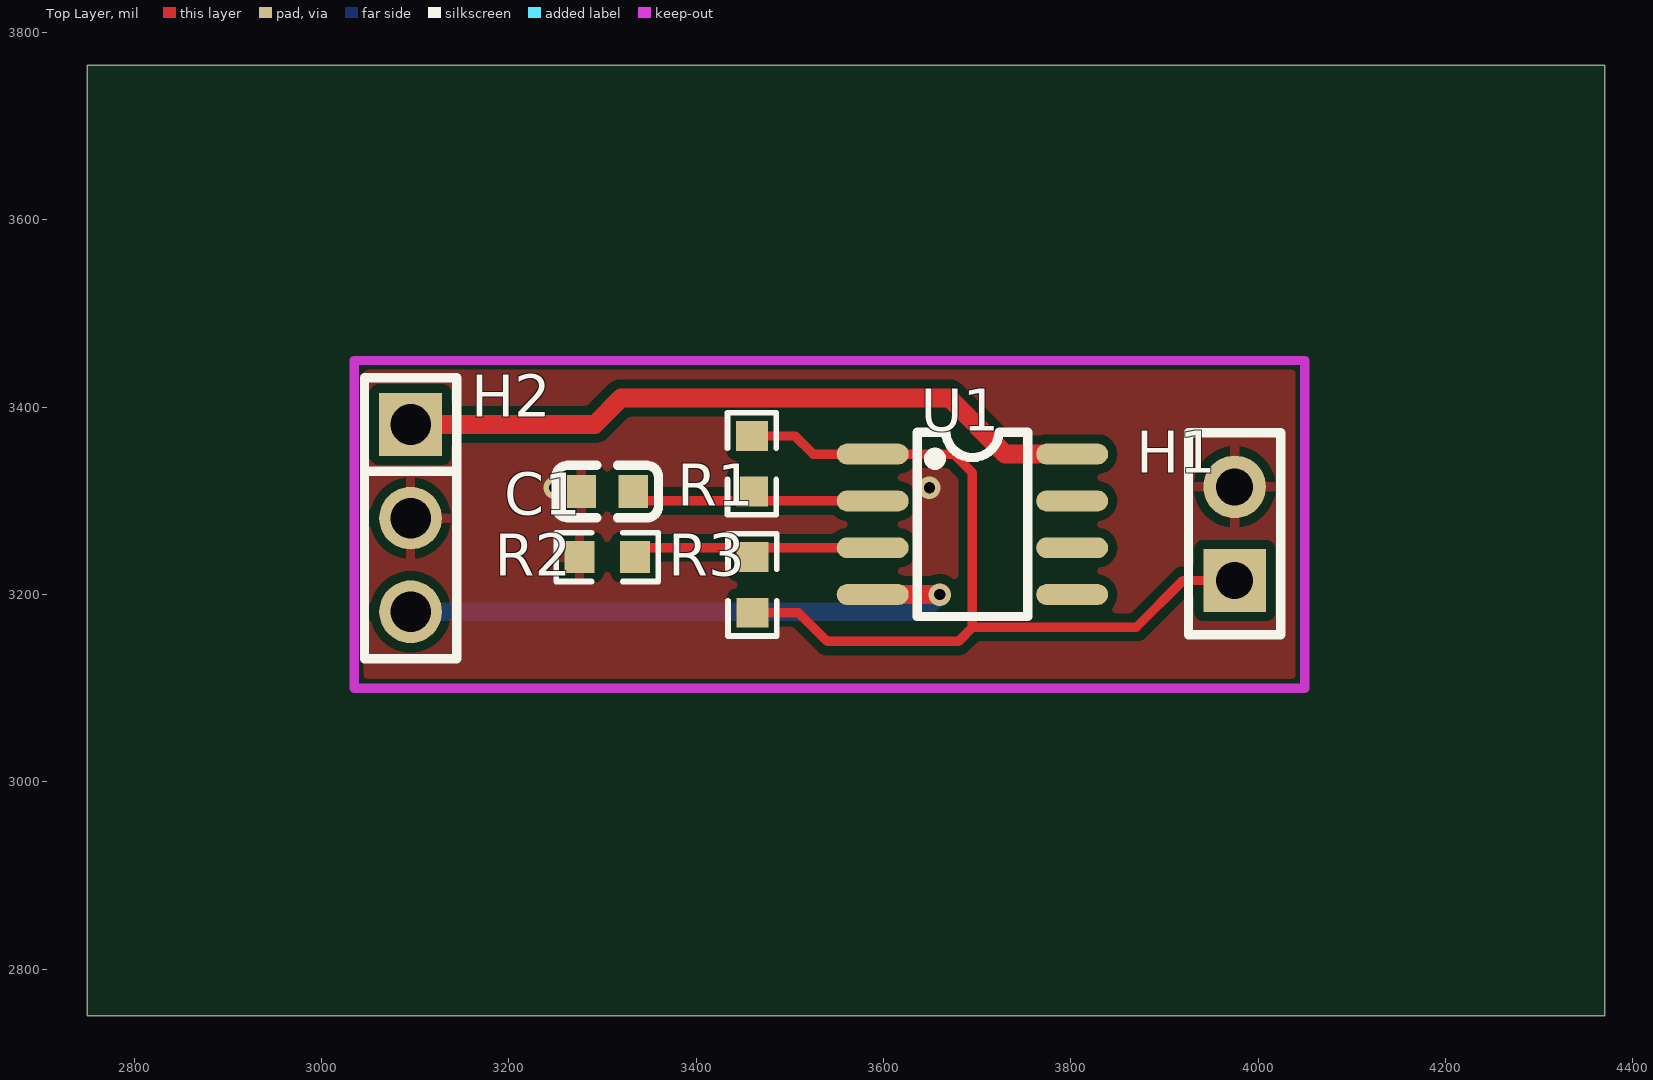
[diagram p0: Top Layer view]
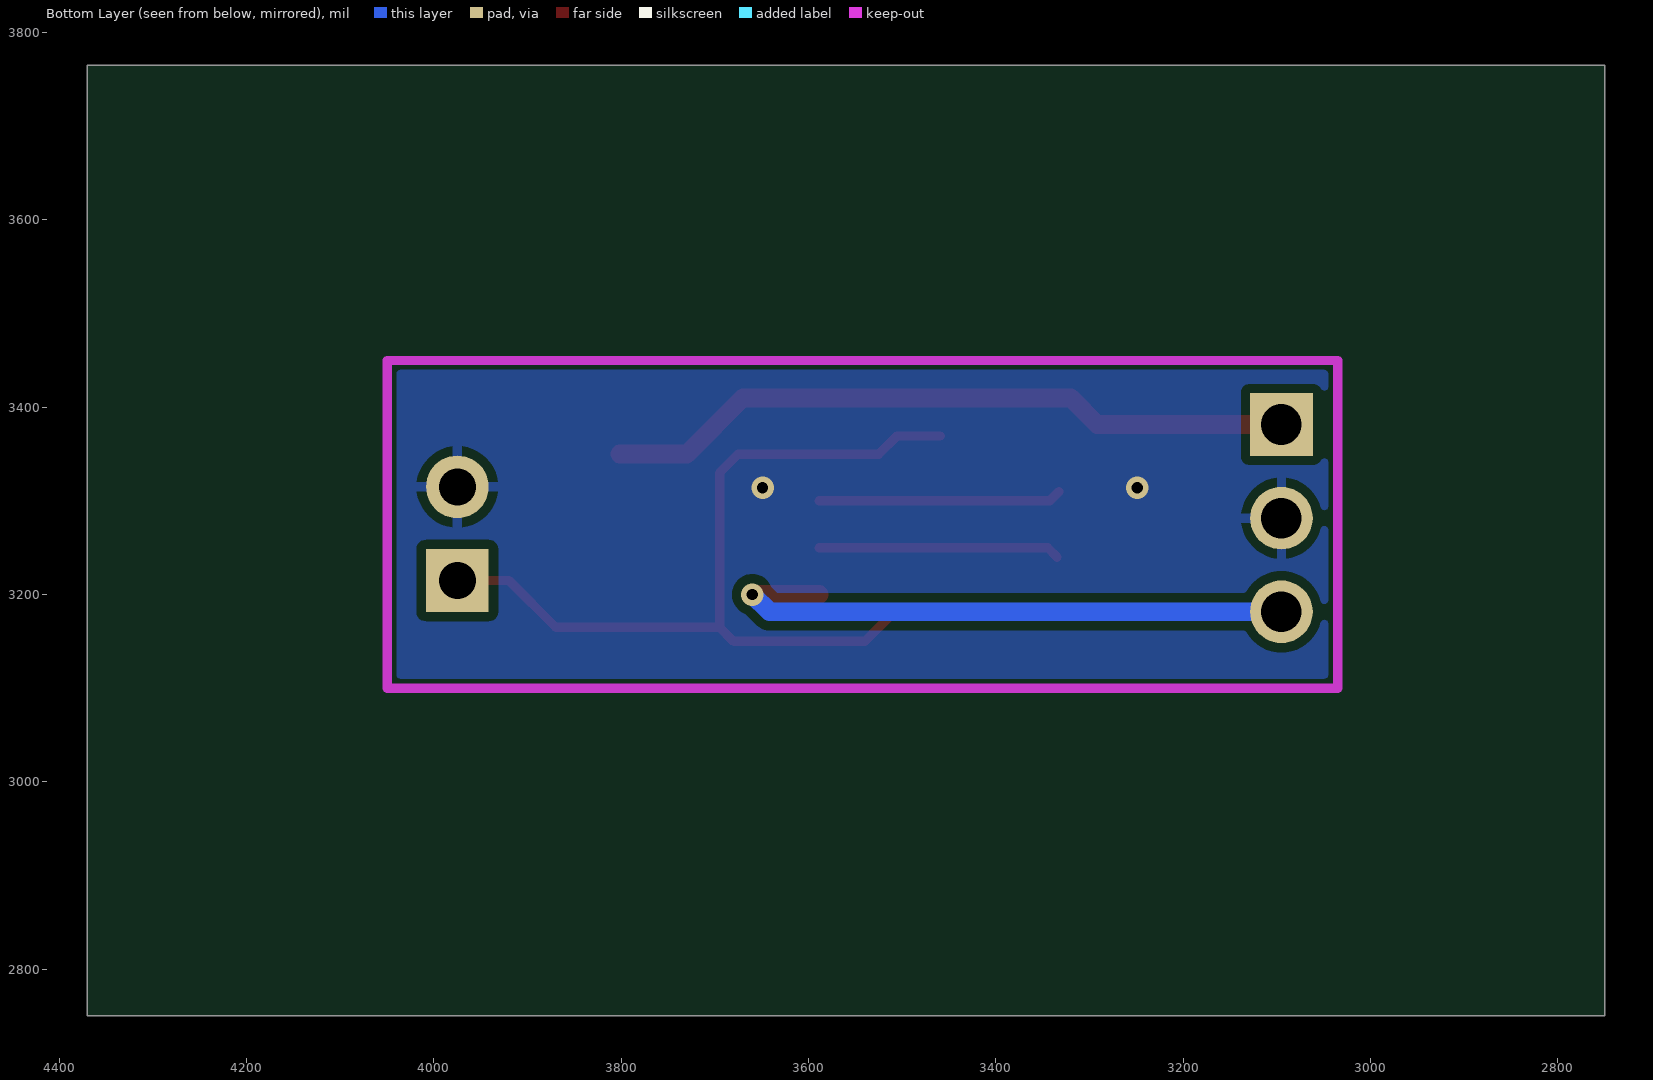
[diagram p1: Bottom Layer view, seen from below]
# Altium PCB MISC89039.pcbdoc
Units mil, origin at the board's own origin, x right, y up, seen from the top; angles counter-clockwise.
Board outline 1620 x 1015 mil, 2 copper layers (Top Layer, Bottom Layer), stack 62.206 mil thick; 7 components, 6 nets, 21 pads, 3 vias.

## Layer stack, top to bottom
Top Solder Mask Layer: solder mask 0.394, Dk 3.3
Top Layer: signal copper 1.379
Dielectric1: surface 59.449, FR4, Dk 4.5
Bottom Layer: signal copper 1.378
Bottom Solder Mask Layer: solder mask 0.394, Dk 3.3

## Board outline
4370,2750 2750,2750 2750,3765 4370,3765

## Design rules (kind name [scope] priority, off if disabled: settings)
BoardOutlineClearance copperThickness2oz_1 [All] p2 off: genericclearance=7.99 ignorepadtopadclearanceinfootprint=FALSE except(0: Arc-SplitContinuation Track-SplitContinuation SMDPad-SplitContinuation THPad-SplitContinuation Via-SplitContinuation Fill-SplitContinuation Region-SplitContinuation Poly-SplitContinuation Text-SplitContinuation Hole-SplitContinuation; 5.98: Arc-CutoutEdge SMDPad-CutoutEdge THPad-CutoutEdge Via-CutoutEdge Fill-CutoutEdge Region-CutoutEdge Text-CutoutEdge; 6.93: Hole-OutlineEdge Hole-CutoutEdge; 10: Poly-OutlineEdge Poly-CutoutEdge; 11.81: Arc-OutlineEdge Track-OutlineEdge SMDPad-OutlineEdge THPad-OutlineEdge Via-OutlineEdge Fill-OutlineEdge Region-OutlineEdge Text-OutlineEdge Track-CutoutEdge)
BoardOutlineClearance copperThickness1oz_1 [All] p4: genericclearance=4.02 ignorepadtopadclearanceinfootprint=FALSE except(0: Arc-SplitContinuation Track-SplitContinuation SMDPad-SplitContinuation THPad-SplitContinuation Via-SplitContinuation Fill-SplitContinuation Region-SplitContinuation Poly-SplitContinuation Text-SplitContinuation Hole-SplitContinuation; 6: SMDPad-CutoutEdge THPad-CutoutEdge Via-CutoutEdge Fill-CutoutEdge Region-CutoutEdge Text-CutoutEdge; 6.93: Hole-OutlineEdge Hole-CutoutEdge; 10: Poly-OutlineEdge Poly-CutoutEdge; 11.8: Arc-OutlineEdge Track-OutlineEdge SMDPad-OutlineEdge THPad-OutlineEdge Via-OutlineEdge Fill-OutlineEdge Region-OutlineEdge Text-OutlineEdge; 11.81: Arc-CutoutEdge Track-CutoutEdge)
Clearance copperThickness2oz [All] p1 off: gap=7.99 ignorepadtopadclearanceinfootprint=FALSE except(5.98: SMDPad-Track SMDPad-SMDPad THPad-Track SMDPad-THPad THPad-THPad Track-Via SMDPad-Via THPad-Via Via-Via Fill-Track Region-Track Fill-SMDPad Region-SMDPad Fill-THPad Region-THPad Fill-Via Region-Via Fill-Fill Fill-Region Region-Region Arc-Track Arc-SMDPad Arc-THPad Arc-Via Fill-Arc Region-Arc Arc-Arc Text-Track SMDPad-Text Text-THPad Text-Via Fill-Text Region-Text Arc-Text Text-Text; 6.93: Hole-Track Hole-SMDPad Hole-THPad Hole-Via Fill-Hole Region-Hole Hole-Arc Hole-Text; 10: Poly-Track Poly-SMDPad Poly-THPad Poly-Via Poly-Fill Poly-Region Poly-Poly Poly-Arc Poly-Text Poly-Hole)
Clearance copperThickness1oz [All] p3: gap=4.02 ignorepadtopadclearanceinfootprint=FALSE except(5.98: SMDPad-Track SMDPad-SMDPad THPad-Track SMDPad-THPad THPad-THPad Track-Via SMDPad-Via THPad-Via Via-Via Fill-Track Region-Track Fill-SMDPad Region-SMDPad Fill-THPad Region-THPad Fill-Via Region-Via Fill-Fill Fill-Region Region-Region; 6: Arc-Track Arc-SMDPad Arc-THPad Arc-Via Fill-Arc Region-Arc Arc-Arc Text-Track SMDPad-Text Text-THPad Text-Via Fill-Text Region-Text Arc-Text Text-Text; 6.93: Hole-Track Hole-SMDPad Hole-THPad Hole-Via Fill-Hole Region-Hole Hole-Arc Hole-Text; 10: Poly-Track Poly-SMDPad Poly-THPad Poly-Via Poly-Fill Poly-Region Poly-Poly Poly-Arc Poly-Text Poly-Hole)
DiffPairsRouting differentialPair [All] p1: maxlimit=6 minlimit=6 mostfreqgap=6 toplayer_minwidth=5 toplayer_prefwidth=10 toplayer_maxwidth=100 toplayer_mingap=6 toplayer_prefgap=6 toplayer_maxgap=6 bottomlayer_minwidth=5 bottomlayer_prefwidth=10 bottomlayer_maxwidth=100 bottomlayer_mingap=6 bottomlayer_prefgap=6 bottomlayer_maxgap=6 maxuncoupledlength=10
HoleToHoleClearance otherClearance [All] p1: gap=11.81 allowstackedmicrovias=TRUE
Length netLength [All] p1: minlimit=0 maxlimit=0
MatchedLengths netLengthTolerance [All] p1: tolerance=1000
PasteMaskExpansion pasteMaskExpansion [All] p1: expansion=0
PlaneConnect innerPlane [All] p1: planeconnectstyle=Relief reliefexpansion=20 reliefentries=4 reliefconductorwidth=10 reliefairgap=10
PolygonConnect copperRegion [(InNet('GND'))] p1: connectstyle=Relief reliefconductorwidth=10 reliefentries=4 polygonreliefangle="90 Angle" airgapwidth=10 via.connectstyle=Relief via.reliefconductorwidth=10 via.reliefentries=4 via.polygonreliefangle="90 Angle" via.airgapwidth=10
RoutingVias viaSize [All] p1: holewidth=12.01 width=24.02 viastyle="Through Hole" minholewidth=11.81 minwidth=19.68 maxholewidth=248.03 maxwidth=393.7
SolderMaskExpansion solderMaskExpansion [IsVia] p1: expansion=-1000 istentingtop=TRUE
SolderMaskExpansion solderMaskExpansion [All] p2: expansion=2 istentingtop=FALSE
Width copperThickness2oz_2 [All] p1 off: maxlimit=100 minlimit=8 preferedwidth=10
Width copperThickness1oz_2 [All] p2: maxlimit=100 minlimit=5 preferedwidth=10

## Components (designator, comment, footprint, x,y, rotation, side; value= is the part's Value field where it differs from the comment)
C1 "100nF" C0603 3305,3310 r0 top
H1 "" HDR-TH_2P-P2.54-V-F 3975,3265 r90 top
H2 "" HDR-TH_3P-P2.54-V-M 3095,3281.61 r270 top
R1 "10K" R0603 3459.45,3339.66 r90 top
R2 "10K" R0603 3305,3240 r0 top
R3 "10K" R0603 3460,3210.34 r270 top
U1 "NE5532DRG4" SOIC-8_L5.0-W4.0-P1.27-LS6.0-BL 3695,3275 r270 top

## Footprints (in the part's own frame and the unit in brackets; to place one, negate y for a bottom-side part, rotate by r counter-clockwise, add the part's x,y. Pads: shape width x height; smd on the part's side, far side on the other; paste and mask are expansions set on the pad)
C0603 [mm]
  rect 0.8x0.9 smd: 1(-0.7,0) 2(0.7,0)
  silkscreen extent -1.39,-0.71 1.39,0.71
HDR-TH_2P-P2.54-V-F [mm]
  rect 1.7x1.7 hole 1: 1(-1.27,0)
  round 1.7 hole 1: 2(1.27,0)
  silkscreen extent -2.74,-1.25 2.74,1.25
HDR-TH_3P-P2.54-V-M [mm]
  rect 1.7x1.7 hole 1.1: 1(-2.54,0)
  round 1.7 hole 1.1: 2(0,0) 3(2.54,0)
  silkscreen extent -3.81,-1.25 3.81,1.25
R0603 [mil]
  rect 31.75x34.02 smd paste-3937.01 mask+2: 1(-29.66,0) 2(29.66,0)
  silkscreen extent -55,-26 55,26
SOIC-8_L5.0-W4.0-P1.27-LS6.0-BL [mil]
  oval 22.38x76.78 smd: 1(-75,-106.5) 2(-25,-106.5) 3(25,-106.5) 4(75,-106.5) 5(75,106.5) 6(25,106.5) 7(-25,106.5) 8(-75,106.5)
  silkscreen extent -98,-59 98,59

## Via types
v1: diameter 24.02, hole 12, Top Layer to Bottom Layer, 3 vias

## Nets (pads, with @x,y where several pads share a name; then routed paths per layer and width w, separated by ;. In a path a pad name is that pad's centre, name@x,y a point inside that pad or via, vN(x,y) a via of type N, cw(c..) or ccw(c..) an arc to the next point about the centre after c; other vN are vias at no path point)
$1N2: C1.2 R1.1 U1.2 | length 260.1
  Top Layer w10: C1.2 3342.56,3300 U1.2
$1N3: R2.2 R3.1 U1.3 | length 258
  Top Layer w10: R2.2 3344.66,3250 U1.3
-VCC: H2.3 U1.4 | length 644.1
  Top Layer w20: U1.4 v1(3660,3200)
  Bottom Layer w20: H2.3 3641.61,3181.61 v1(3660,3200)
GND: C1.1 H1.2 H2.2 R2.1
  other v1: 3249.1,3314.1 3649.1,3314.1
VCC: H2.1 U1.8 | length 743.1
  Top Layer w20: H2.1 3291.61,3381.61 3320,3410 3670,3410 3730,3350 U1.8
VO: H1.1 R1.2 R3.2 U1.1 | length 971.5
  Top Layer w10: R1.2 3505.68,3369.32 3525,3350 U1.1 3675,3350 3695,3330 3695,3165 ; R3.2 3509.32,3180.68 3540,3150 3680,3150 3695,3165 ; H1.1 3920,3215 3870,3165 3695,3165
pads on no net: U1.5 U1.6 U1.7

## Polygon pours and split planes (outlines as drawn)
GND on Top Layer (solid, remove dead copper, pour order 0): 3000,3515 3000,3000 4120,3000 4120,3515
GND on Bottom Layer (solid, remove dead copper, pour order 2): 3015,3485 3015,3055 4095,3055 4095,3485

## Keep-outs
Board Outline Layer:
  lines w10: 3035,3100 3035,3450 4050,3450 4050,3100 3035,3100